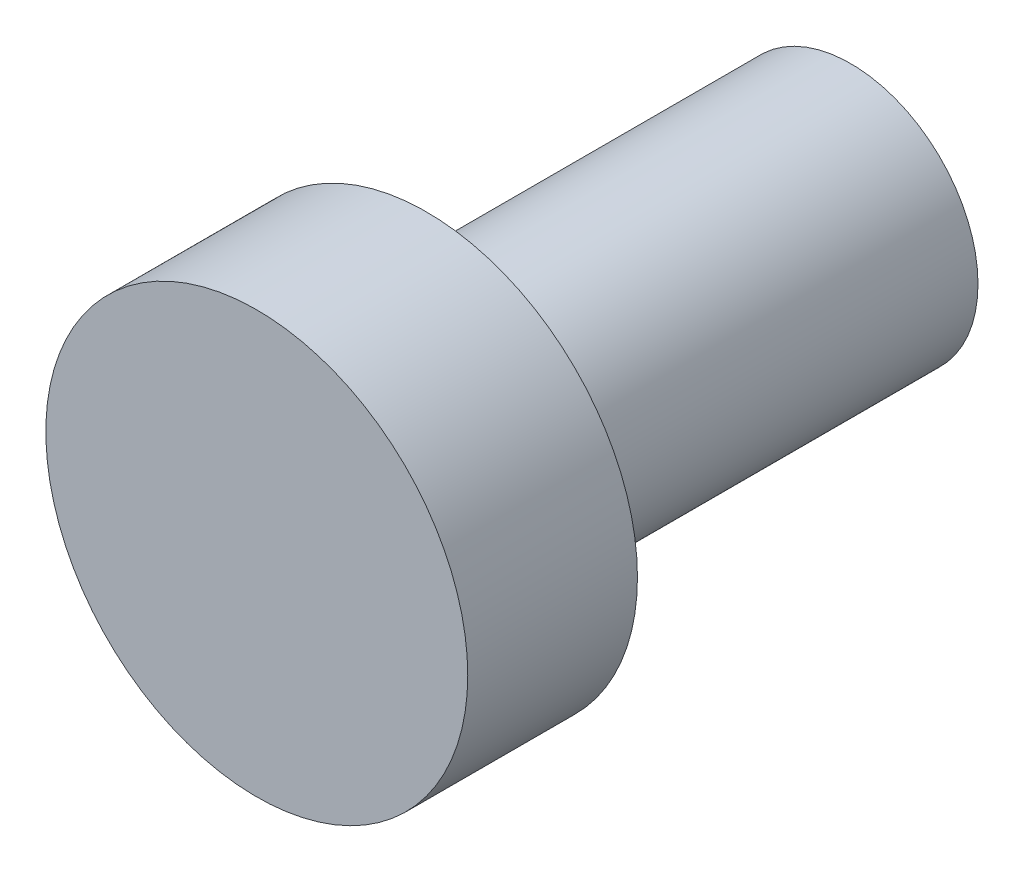
from build123d import *

# Parameters (mm, degrees)
SKETCH1_R           = 1.5
BOSS_EXTRUDE1_DEPTH = 5
SKETCH2_R           = 2.486398422
BOSS_EXTRUDE2_DEPTH = 2


with BuildPart() as part:
    # Sketch1 → Boss-Extrude1 (new body)
    with BuildSketch(Plane.XY):
        with Locations((45.197762361, 32.025823543)):
            Circle(SKETCH1_R)
    extrude(amount=-BOSS_EXTRUDE1_DEPTH)

    # Sketch2 → Boss-Extrude2 (add)
    with BuildSketch(Plane.XY):
        with Locations((45.197762361, 32.025823543)):
            Circle(SKETCH2_R)
    extrude(amount=BOSS_EXTRUDE2_DEPTH)


solid = part.part
